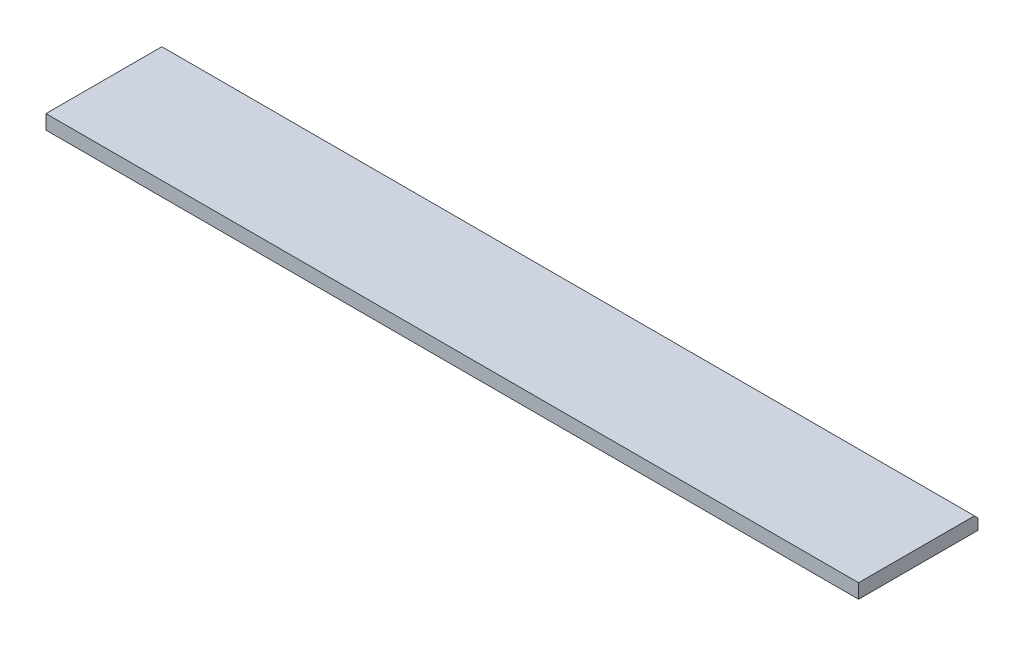
SolidWorks part; units mm, degrees
ref_plane "前视基准面" through (0, 0, 0) normal (0, 0, 1) x (1, 0, 0)
ref_plane "上视基准面" through (0, 0, 0) normal (0, 1, 0) x (1, 0, 0)
ref_plane "右视基准面" through (0, 0, 0) normal (1, 0, 0) x (0, 0, -1)
sketch "草图1" plane through (0, 0, 0) normal (0, 1, 0) x (1, 0, 0)
  line L1 (-1133, -166.5) -> (1133, -166.5)
  line L2 (-1133, -166.5) -> (-1133, 166.5)
  line L3 (-1133, 166.5) -> (1133, 166.5)
  line L4 (1133, -166.5) -> (1133, 166.5)
  line L5 (-1133, -166.5) -> (1133, 166.5) construction
  line L6 (-1133, 166.5) -> (1133, -166.5) construction
  point P0 (0, 0)
  dimension "D1" = 333
  dimension "D2" = 2266
extrude "凸台-拉伸1" add sketch "草图1" along normal blind 40
chamfer "倒角1" distance 10 angle 45 1 edges at (0, 40, -166.5)
